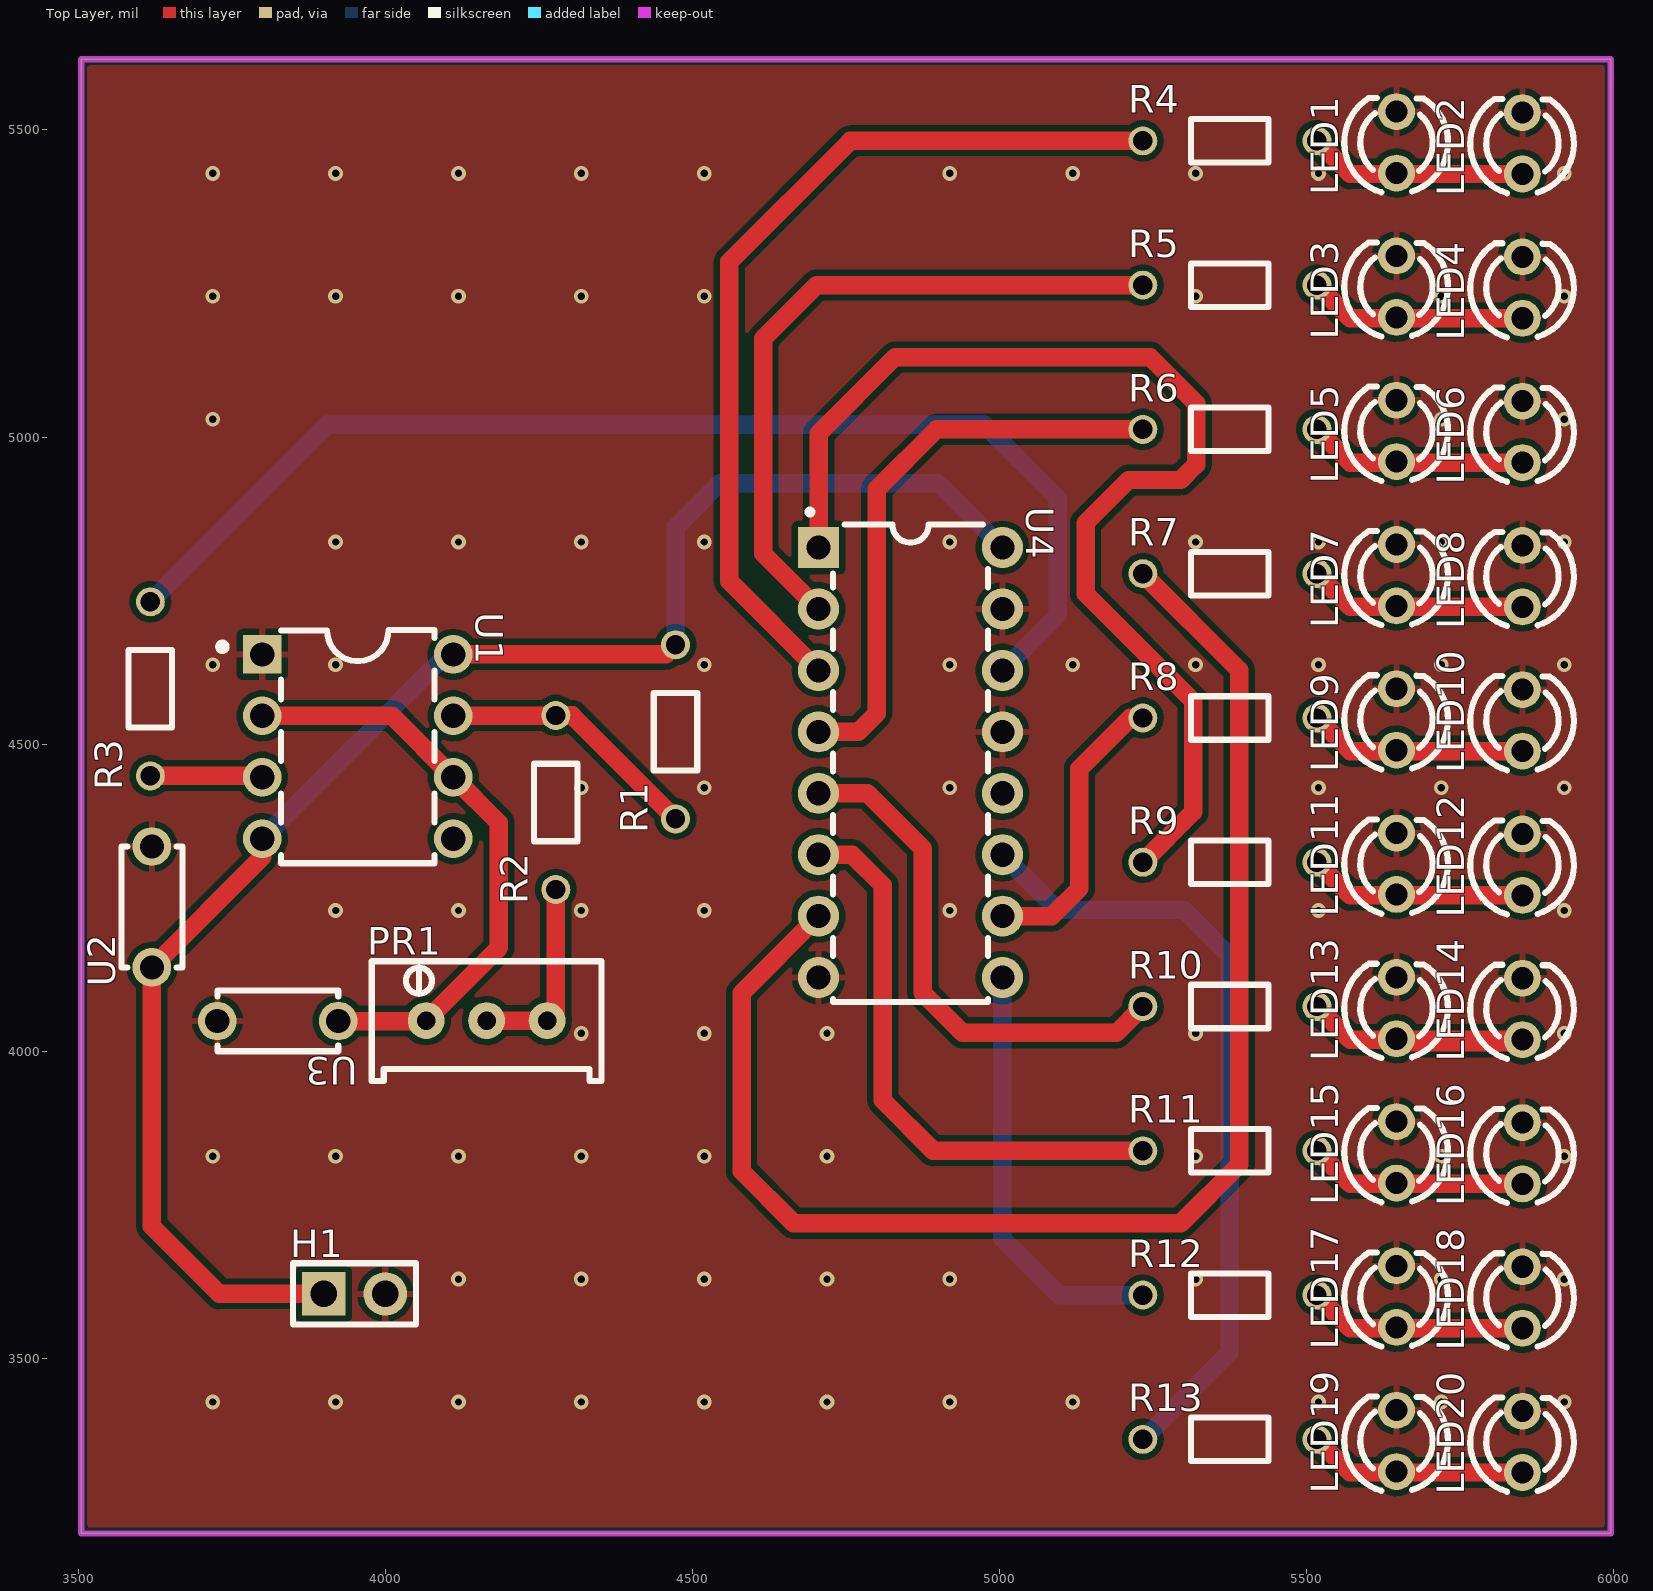
[diagram p0: Top Layer view]
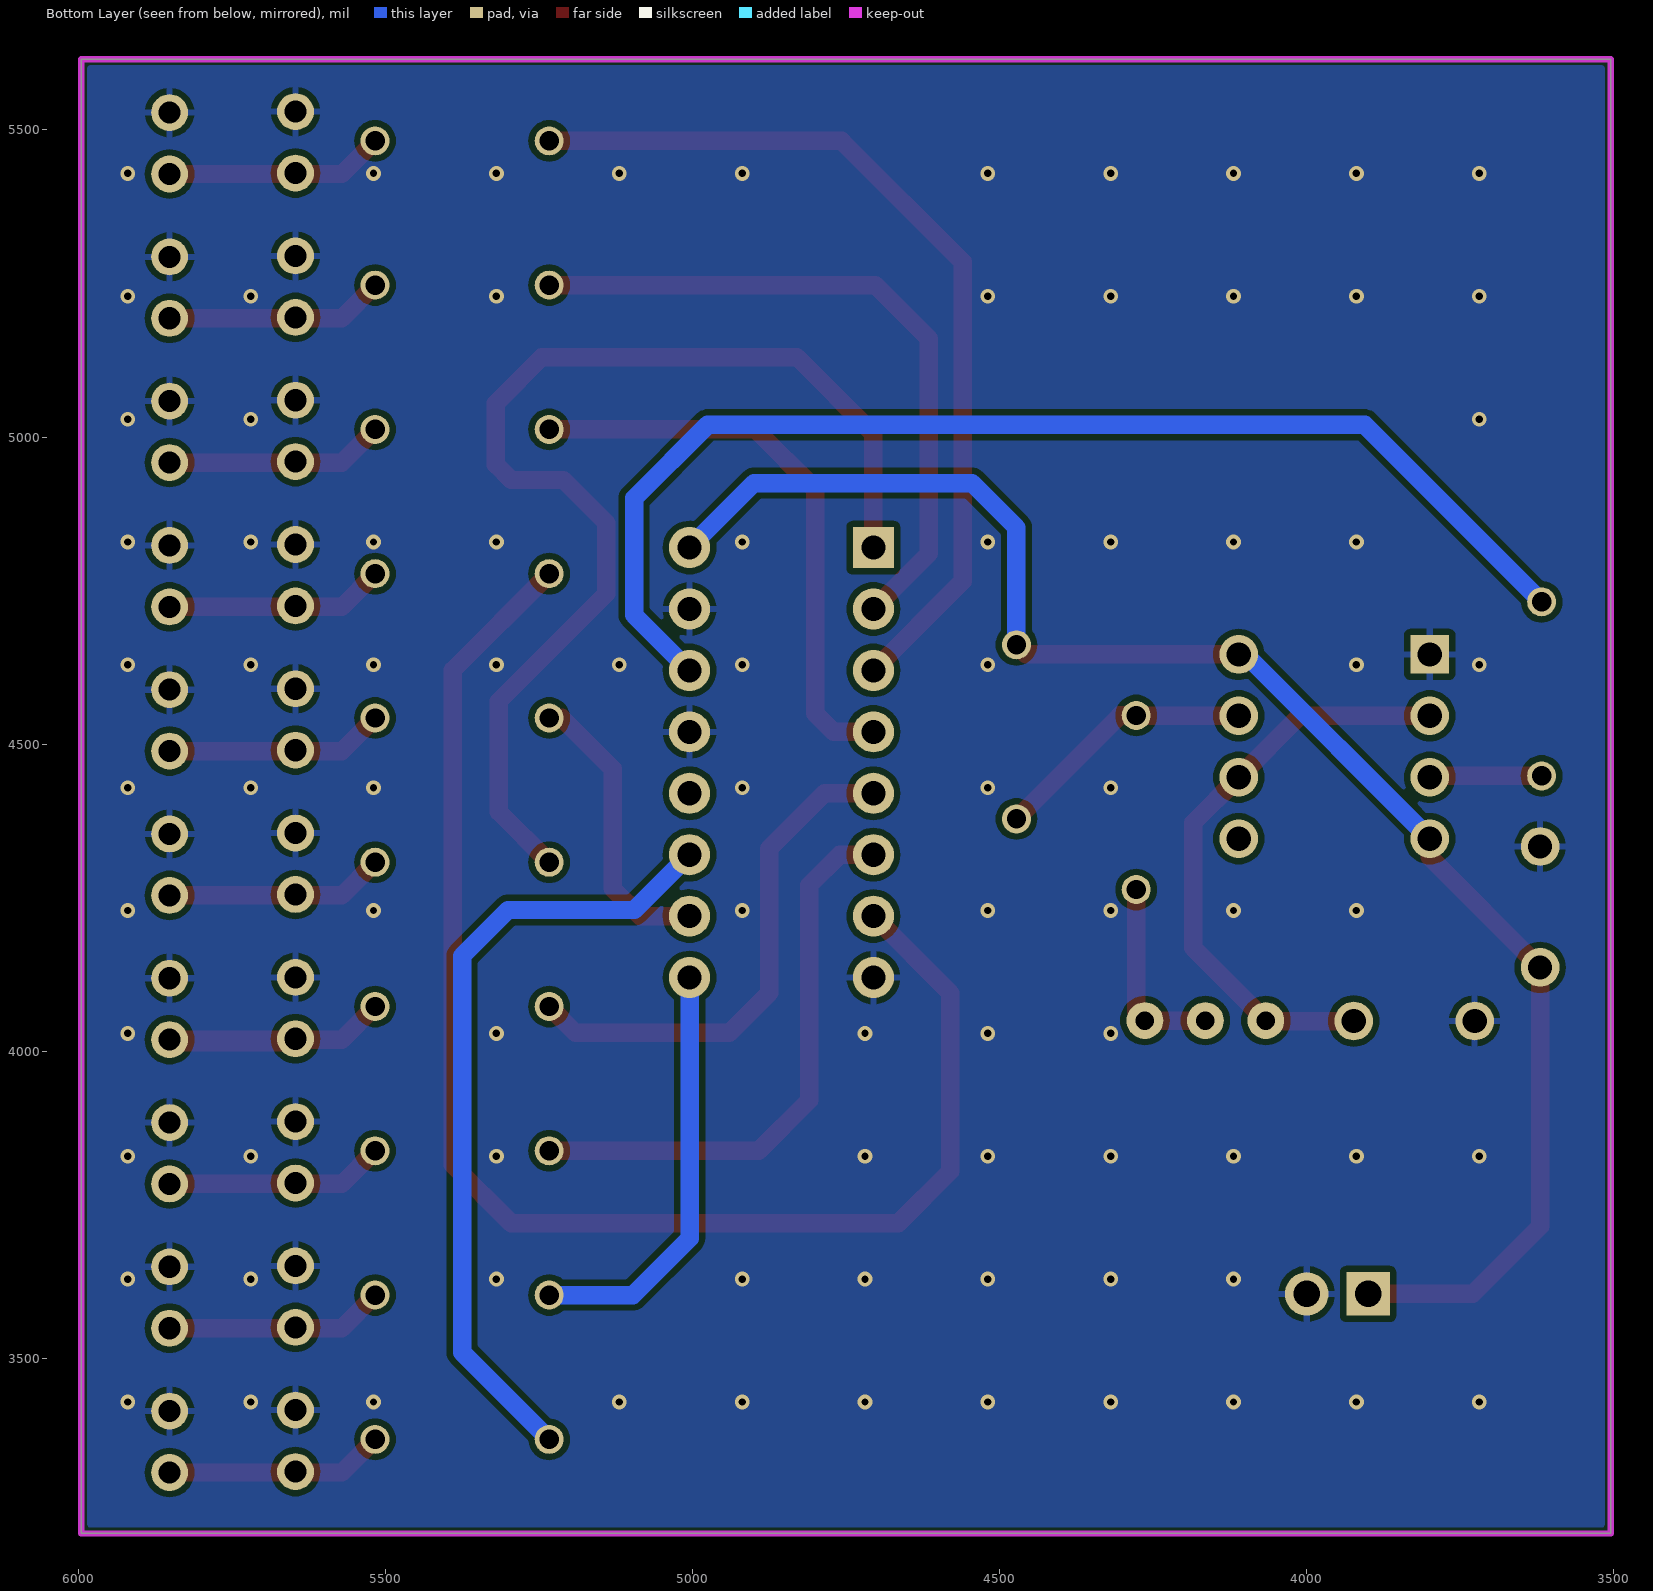
[diagram p1: Bottom Layer view, seen from below]
# Altium PCB MISC51889.pcbdoc
Units mil, origin at the board's own origin, x right, y up, seen from the top; angles counter-clockwise.
Board outline 2490 x 2400 mil, 2 copper layers (Top Layer, Bottom Layer), stack 62.206 mil thick; 39 components, 27 nets, 99 pads, 85 vias.

## Layer stack, top to bottom
Top Solder Mask Layer: solder mask 0.394, Dk 3.3
Top Layer: signal copper 1.379
Dielectric1: surface 59.449, FR4, Dk 4.5
Bottom Layer: signal copper 1.378
Bottom Solder Mask Layer: solder mask 0.394, Dk 3.3

## Board outline
3505,5615 3505,3215 5995,3215 5995,5615

## Design rules (kind name [scope] priority, off if disabled: settings)
BoardOutlineClearance copperThickness2oz_1 [All] p2 off: genericclearance=7.99 ignorepadtopadclearanceinfootprint=FALSE except(0: Arc-SplitContinuation Track-SplitContinuation SMDPad-SplitContinuation THPad-SplitContinuation Via-SplitContinuation Fill-SplitContinuation Region-SplitContinuation Poly-SplitContinuation Text-SplitContinuation Hole-SplitContinuation; 5.98: Arc-CutoutEdge SMDPad-CutoutEdge THPad-CutoutEdge Via-CutoutEdge Fill-CutoutEdge Region-CutoutEdge Text-CutoutEdge; 6.93: Hole-OutlineEdge Hole-CutoutEdge; 10: Poly-OutlineEdge Poly-CutoutEdge; 11.81: Arc-OutlineEdge Track-OutlineEdge SMDPad-OutlineEdge THPad-OutlineEdge Via-OutlineEdge Fill-OutlineEdge Region-OutlineEdge Text-OutlineEdge Track-CutoutEdge)
BoardOutlineClearance copperThickness1oz_1 [All] p4: genericclearance=4.02 ignorepadtopadclearanceinfootprint=FALSE except(0: Arc-SplitContinuation Track-SplitContinuation SMDPad-SplitContinuation THPad-SplitContinuation Via-SplitContinuation Fill-SplitContinuation Region-SplitContinuation Poly-SplitContinuation Text-SplitContinuation Hole-SplitContinuation; 6: SMDPad-CutoutEdge THPad-CutoutEdge Via-CutoutEdge Fill-CutoutEdge Region-CutoutEdge Text-CutoutEdge; 6.93: Hole-OutlineEdge Hole-CutoutEdge; 10: Poly-OutlineEdge Poly-CutoutEdge; 11.8: Arc-OutlineEdge Track-OutlineEdge SMDPad-OutlineEdge THPad-OutlineEdge Via-OutlineEdge Fill-OutlineEdge Region-OutlineEdge Text-OutlineEdge; 11.81: Arc-CutoutEdge Track-CutoutEdge)
Clearance copperThickness2oz [All] p1 off: gap=7.99 ignorepadtopadclearanceinfootprint=FALSE except(5.98: SMDPad-Track SMDPad-SMDPad THPad-Track SMDPad-THPad THPad-THPad Track-Via SMDPad-Via THPad-Via Via-Via Fill-Track Region-Track Fill-SMDPad Region-SMDPad Fill-THPad Region-THPad Fill-Via Region-Via Fill-Fill Fill-Region Region-Region Arc-Track Arc-SMDPad Arc-THPad Arc-Via Fill-Arc Region-Arc Arc-Arc Text-Track SMDPad-Text Text-THPad Text-Via Fill-Text Region-Text Arc-Text Text-Text; 6.93: Hole-Track Hole-SMDPad Hole-THPad Hole-Via Fill-Hole Region-Hole Hole-Arc Hole-Text; 10: Poly-Track Poly-SMDPad Poly-THPad Poly-Via Poly-Fill Poly-Region Poly-Poly Poly-Arc Poly-Text Poly-Hole)
Clearance copperThickness1oz [All] p3: gap=4.02 ignorepadtopadclearanceinfootprint=FALSE except(5.98: SMDPad-Track SMDPad-SMDPad THPad-Track SMDPad-THPad THPad-THPad Track-Via SMDPad-Via THPad-Via Via-Via Fill-Track Region-Track Fill-SMDPad Region-SMDPad Fill-THPad Region-THPad Fill-Via Region-Via Fill-Fill Fill-Region Region-Region; 6: Arc-Track Arc-SMDPad Arc-THPad Arc-Via Fill-Arc Region-Arc Arc-Arc Text-Track SMDPad-Text Text-THPad Text-Via Fill-Text Region-Text Arc-Text Text-Text; 6.93: Hole-Track Hole-SMDPad Hole-THPad Hole-Via Fill-Hole Region-Hole Hole-Arc Hole-Text; 10: Poly-Track Poly-SMDPad Poly-THPad Poly-Via Poly-Fill Poly-Region Poly-Poly Poly-Arc Poly-Text Poly-Hole)
Creepage creepage [All] p1: checkdistance=0 ignoreinternallayers=TRUE applytopolygonpour=TRUE
DiffPairsRouting differentialPair [All] p1: maxlimit=6 minlimit=6 mostfreqgap=6 toplayer_minwidth=5 toplayer_prefwidth=10 toplayer_maxwidth=100 toplayer_mingap=6 toplayer_prefgap=6 toplayer_maxgap=6 bottomlayer_minwidth=5 bottomlayer_prefwidth=10 bottomlayer_maxwidth=100 bottomlayer_mingap=6 bottomlayer_prefgap=6 bottomlayer_maxgap=6 maxuncoupledlength=10
HoleToHoleClearance otherClearance [All] p1: gap=11.81 allowstackedmicrovias=TRUE
Length netLength [All] p1: minlimit=0 maxlimit=0
MatchedLengths netLengthTolerance [All] p1: tolerance=1000
PasteMaskExpansion pasteMaskExpansion [All] p1: expansion=0
PlaneConnect innerPlane [All] p1: planeconnectstyle=Relief reliefexpansion=20 reliefentries=4 reliefconductorwidth=10 reliefairgap=10
PolygonConnect copperRegion [(InNet('GND'))] p1: connectstyle=Relief reliefconductorwidth=10 reliefentries=4 polygonreliefangle="90 Angle" airgapwidth=10 via.connectstyle=Relief via.reliefconductorwidth=10 via.reliefentries=4 via.polygonreliefangle="90 Angle" via.airgapwidth=10
RoutingVias viaSize [All] p1: holewidth=12.01 width=24.02 viastyle="Through Hole" minholewidth=11.81 minwidth=19.68 maxholewidth=248.03 maxwidth=393.7
SolderMaskExpansion solderMaskExpansion [IsVia] p1: expansion=-1000 istentingtop=TRUE
SolderMaskExpansion solderMaskExpansion [All] p2: expansion=2 istentingtop=FALSE
Width copperThickness2oz_2 [All] p1 off: maxlimit=100 minlimit=8 preferedwidth=10
Width copperThickness1oz_2 [All] p2: maxlimit=100 minlimit=5 preferedwidth=10

## Components (designator, comment, footprint, x,y, rotation, side; value= is the part's Value field where it differs from the comment)
H1 "" HDR-TH_2P-P2.54-V-M-1 3950,3605 r0 top
LED1 "" LED_TH-3mm 5646.17,5479.65 r90 top
LED2 "" LED_TH-3mm 5851.17,5478.15 r90 top
LED3 "" LED_TH-3mm 5646.17,5244.77 r90 top
LED4 "" LED_TH-3mm 5851.17,5243.27 r90 top
LED5 "" LED_TH-3mm 5646.17,5009.9 r90 top
LED6 "" LED_TH-3mm 5851.17,5008.4 r90 top
LED7 "" LED_TH-3mm 5646.17,4775.02 r90 top
LED8 "" LED_TH-3mm 5851.17,4773.52 r90 top
LED9 "" LED_TH-3mm 5646.17,4540.14 r90 top
LED10 "" LED_TH-3mm 5851.17,4538.65 r90 top
LED11 "" LED_TH-3mm 5646.17,4305.27 r90 top
LED12 "" LED_TH-3mm 5851.17,4303.77 r90 top
LED13 "" LED_TH-3mm 5646.17,4070.39 r90 top
LED14 "" LED_TH-3mm 5851.17,4068.89 r90 top
LED15 "" LED_TH-3mm 5646.17,3835.52 r90 top
LED16 "" LED_TH-3mm 5851.17,3834.02 r90 top
LED17 "" LED_TH-3mm 5646.17,3600.64 r90 top
LED18 "" LED_TH-3mm 5851.17,3599.14 r90 top
LED19 "" LED_TH-3mm 5646.17,3365.76 r90 top
LED20 "" LED_TH-3mm 5851.17,3364.26 r90 top
PR1 "10kΩ" R_3296 4165,4055 r0 top
R1 "2.2kΩ" Res_1/8W 4475,4520 r90 top
R2 "10kΩ" Res_1/8W 4280,4405 r90 top
R3 "10kΩ" Res_1/8W 3620,4590 r90 top
R4 "10Ω" Res_1/8W 5374.92,5479.65 r0 top
R5 "10Ω" Res_1/8W 5374.92,5244.77 r0 top
R6 "10Ω" Res_1/8W 5374.92,5009.9 r0 top
R7 "10Ω" Res_1/8W 5374.92,4775.02 r0 top
R8 "10Ω" Res_1/8W 5374.92,4540.14 r0 top
R9 "10Ω" Res_1/8W 5374.92,4305.27 r0 top
R10 "10Ω" Res_1/8W 5374.92,4070.39 r0 top
R11 "10Ω" Res_1/8W 5374.92,3835.52 r0 top
R12 "10Ω" Res_1/8W 5374.92,3600.64 r0 top
R13 "10Ω" Res_1/8W 5374.92,3365.76 r0 top
U1 "NE555PE4" PDIP-8_L9.6-W6.4-P2.54-LS7.9-BL-1 3955.21,4496.1 r270 top
U2 "100nF" CAP-TH_L5.0-W2.5-P5.00-D1.0 3620,4235 r90 top
U3 "1uF" CAP-TH_L5.0-W2.5-P5.00-D1.0 3825,4049.21 r180 top
U4 "4017BDM" PDIP-16_L19.3-W6.5-P2.54-LS7.6-BL 4855,4470 r270 top

## Footprints (in the part's own frame and the unit in brackets; to place one, negate y for a bottom-side part, rotate by r counter-clockwise, add the part's x,y. Pads: shape width x height; smd on the part's side, far side on the other; paste and mask are expansions set on the pad)
CAP-TH_L5.0-W2.5-P5.00-D1.0 [mm]
  round 1.6 hole 1: 1(-2.5,0) 2(2.5,0)
  silkscreen extent -2.5,-1.27 2.5,1.25
HDR-TH_2P-P2.54-V-M-1 [mm]
  rect 1.8x1.8 hole 1.1: 1(-1.27,0)
  round 1.8 hole 1.1: 2(1.27,0)
  silkscreen extent -2.54,-1.27 2.54,1.27
LED_TH-3mm [mil]
  round 60 hole 36 paste+0 mask+2: 1(-50,0) 2(50,0)
  silkscreen extent -81,-84 72,85
PDIP-8_L9.6-W6.4-P2.54-LS7.9-BL-1 [mil]
  rect 63x63 hole 39.37: 1(-150,-155.51)
  round 63 hole 39.37: 2(-50,-155.51) 3(50,-155.51) 4(150,-155.51) 5(150,155.52) 6(50,155.52) 7(-50,155.52) 8(-150,155.52)
  silkscreen extent -190,-226 190,125
PDIP-16_L19.3-W6.5-P2.54-LS7.6-BL [mm]
  rect 1.7x1.7 hole 1: 1(-8.89,-3.8)
  round 1.7 hole 1: 2(-6.35,-3.8) 3(-3.81,-3.8) 4(-1.27,-3.8) 5(1.27,-3.8) 6(3.81,-3.8) 7(6.35,-3.8) 8(8.89,-3.8) 9(8.89,3.8) 10(6.35,3.8) 11(3.81,3.8) 12(1.27,3.8) 13(-1.27,3.8) 14(-3.81,3.8) 15(-6.35,3.8) 16(-8.89,3.8)
  silkscreen extent -10.46,-4.26 9.9,3.2
R_3296 [mil]
  round 60 hole 30 paste+0 mask+2: 1(-98.4,-5) 2(0,-5) 3(98.4,-5)
  silkscreen extent -187,-103 187,92
Res_1/8W [mil]
  round 47.2 hole 31.5 paste+0 mask+2: 1(-141.7,2.48) 2(141.7,2.48)
  silkscreen extent -63,-33 63,38

## Via types
v1: diameter 24.02, hole 12, Top Layer to Bottom Layer, 85 vias

## Nets (pads, with @x,y where several pads share a name; then routed paths per layer and width w, separated by ;. In a path a pad name is that pad's centre, name@x,y a point inside that pad or via, vN(x,y) a via of type N, cw(c..) or ccw(c..) an arc to the next point about the centre after c; other vN are vias at no path point)
$1N1: H1.1 R1.2 U1.4 U1.8 U2.1 U4.16 | length 2631.1
  Top Layer w30: U1.4 3799.7,4316.27 U2.1 3620,3715 3730,3605 H1.1 ; U1.8 4456.93,4646.1 R1.2
  Bottom Layer w30: U1.4 4099.7,4646.1 U1.8 ; R1.2 4472.52,4852.52 4545,4925 4899.61,4925 U4.16
$1N4: R1.1 R2.2 U1.7 | length 431.8
  Top Layer w30: U1.7 4276.93,4546.1 R2.2 4304.12,4546.7 R1.1
$1N5: PR1.1 U1.2 U1.6 U3.1 | length 971.9
  Top Layer w30: U1.2 4010.72,4546.1 U1.6 4185,4371.82 4185,4168.4 PR1.1 4065.81,4049.21 U3.1
$1N7: PR1.2 PR1.3 R2.1 | length 317.6
  Top Layer w30: PR1.2 PR1.3 4277.52,4064.12 R2.1
$1N9: R3.1 U1.3 | length 183.1
  Top Layer w30: R3.1 3797.5,4448.3 U1.3
$1N10: R3.2 U4.14 | length 1964
  Bottom Layer w30: R3.2 3905.82,5020 4975,5020 5095,4900 5095,4710.39 U4.14
$1N12: LED1.1 LED2.1 R4.2 | length 356.9
  Top Layer w30: R4.2 5570.6,5428.15 LED2.1
$1N14: LED3.1 LED4.1 R5.2 | length 356.9
  Top Layer w30: R5.2 5570.6,5193.27 LED4.1
$1N15: LED5.1 LED6.1 R6.2 | length 356.9
  Top Layer w30: R6.2 5570.6,4958.4 LED6.1
$1N16: LED7.1 LED8.1 R7.2 | length 356.9
  Top Layer w30: R7.2 5570.6,4723.52 LED8.1
$1N17: LED9.1 LED10.1 R8.2 | length 356.9
  Top Layer w30: R8.2 5570.6,4488.65 LED10.1
$1N18: LED11.1 LED12.1 R9.2 | length 356.9
  Top Layer w30: R9.2 5570.6,4253.77 LED12.1
$1N19: LED13.1 LED14.1 R10.2 | length 561.9
  Top Layer w30: R10.2 5570.6,4018.89 LED14.1 ; LED13.1@5646.17,4015 LED14.1@5851.17,4015
$1N20: LED15.1 LED16.1 R11.2 | length 356.9
  Top Layer w30: R11.2 5570.6,3784.02 LED16.1
$1N21: LED17.1 LED18.1 R12.2 | length 356.9
  Top Layer w30: R12.2 5570.6,3549.14 LED18.1
$1N22: LED19.1 LED20.1 R13.2 | length 356.9
  Top Layer w30: R13.2 5570.6,3314.26 LED20.1
$1N23: R4.1 U4.3 | length 1480.1
  Top Layer w30: U4.3 4560,4765.39 4560,5285 4757.13,5482.13 R4.1
$1N24: R5.1 U4.2 | length 1131.8
  Top Layer w30: U4.2 4615,4810.39 4615,5160 4702.25,5247.25 R5.1
$1N25: R6.1 U4.4 | length 945.6
  Top Layer w30: U4.4 4770,4520 4800,4550 4800,4915 4897.37,5012.37 R6.1
$1N26: R7.1 U4.7 | length 2378.9
  Top Layer w30: U4.7 4580,4094.61 4580,3805 4665,3720 5295,3720 5390,3815 5390,4620.72 R7.1
$1N27: R8.1 U4.10 | length 476.5
  Top Layer w30: U4.10 5085,4220 5130,4265 5130,4460 5212.62,4542.62 R8.1
$1N28: R9.1 U4.1 | length 1860.6
  Top Layer w30: U4.1 4705.39,5005.39 4830,5130 5245,5130 5320,5055 5320,4955 5295,4930 5210,4930 5140,4860 5140,4745 5315,4570 5315,4389.52 R9.1
$1N29: R10.1 U4.5 | length 844.8
  Top Layer w30: U4.5 4785,4420 4875,4330 4875,4095 4940,4030 5190.35,4030 R10.1
$1N30: R11.1 U4.6 | length 932.5
  Top Layer w30: U4.6 4760,4320 4810,4270 4810,3920 4892.01,3837.99 R11.1
$1N31: R12.1 U4.9 | length 691.4
  Bottom Layer w30: U4.9 5004.61,3695.39 5096.88,3603.12 R12.1
$1N32: R13.1 U4.11 | length 1284.2
  Bottom Layer w30: U4.11 5094.61,4230 5300,4230 5375,4155 5375,3510.02 R13.1
GND: H1.2 LED1.2 LED2.2 LED3.2 LED4.2 LED5.2 LED6.2 LED7.2 LED8.2 LED9.2 LED10.2 LED11.2 LED12.2 LED13.2 LED14.2 LED15.2 LED16.2 LED17.2 LED18.2 LED19.2 LED20.2 U1.1 U2.2 U3.2 U4.8 U4.13 U4.15
  other v1: 3719.1,3429.1 3919.1,3429.1 4119.1,3429.1 4319.1,3429.1 4519.1,3429.1 4719.1,3429.1 4919.1,3429.1 5119.1,3429.1 5519.1,3429.1 5719.1,3429.1 5919.1,3429.1 4119.1,3629.1 4319.1,3629.1 4519.1,3629.1 4719.1,3629.1 4919.1,3629.1 5319.1,3629.1 5719.1,3629.1 5919.1,3629.1 3719.1,3829.1 3919.1,3829.1 4119.1,3829.1 4319.1,3829.1 4519.1,3829.1 4719.1,3829.1 5319.1,3829.1 5719.1,3829.1 5919.1,3829.1 4319.1,4029.1 4519.1,4029.1 4719.1,4029.1 5319.1,4029.1 5919.1,4029.1 3919.1,4229.1 4119.1,4229.1 4319.1,4229.1 4519.1,4229.1 4919.1,4229.1 5519.1,4229.1 5919.1,4229.1 4319.1,4429.1 4519.1,4429.1 4919.1,4429.1 5519.1,4429.1 5719.1,4429.1 5919.1,4429.1 3719.1,4629.1 3919.1,4629.1 4519.1,4629.1 4919.1,4629.1 5119.1,4629.1 5319.1,4629.1 5519.1,4629.1 5719.1,4629.1 5919.1,4629.1 3919.1,4829.1 4119.1,4829.1 4319.1,4829.1 4519.1,4829.1 4919.1,4829.1 5319.1,4829.1 5519.1,4829.1 5719.1,4829.1 5919.1,4829.1 3719.1,5029.1 5719.1,5029.1 5919.1,5029.1 3719.1,5229.1 3919.1,5229.1 4119.1,5229.1 4319.1,5229.1 4519.1,5229.1 5319.1,5229.1 5719.1,5229.1 5919.1,5229.1 3719.1,5429.1 3919.1,5429.1 4119.1,5429.1 4319.1,5429.1 4519.1,5429.1 4919.1,5429.1 5119.1,5429.1 5319.1,5429.1 5519.1,5429.1 5919.1,5429.1
pads on no net: U1.5 U4.12

## Polygon pours and split planes (outlines as drawn)
GND on Top Layer (solid, remove dead copper, pour order 0): 3000,5835 3000,3000 6380,3000 6380,5835
GND on Bottom Layer (solid, remove dead copper, pour order 2): 3280,5725 3280,3050 6380,3050 6380,5725

## Keep-outs
Board Outline Layer:
  the board outline again, w10